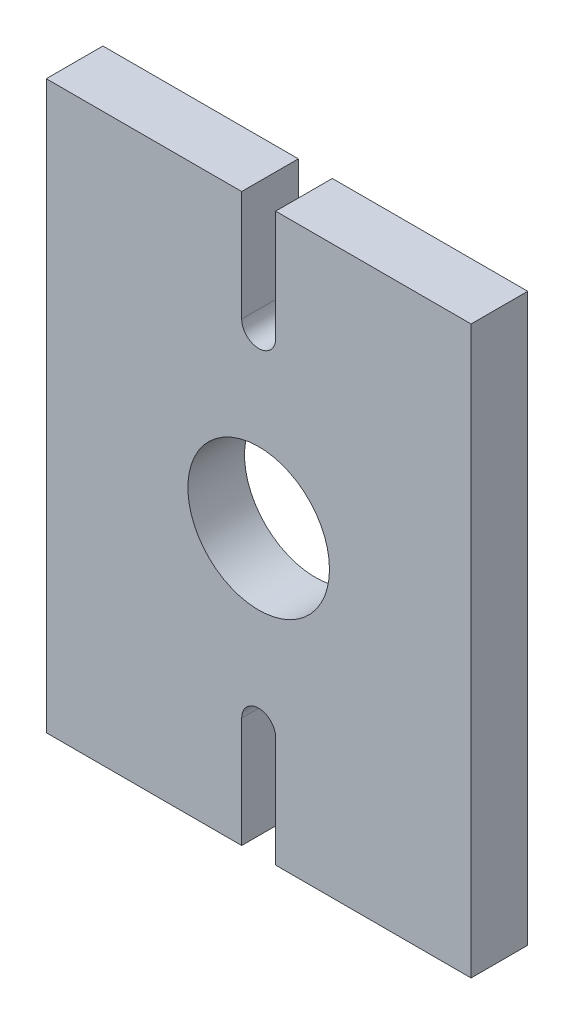
from build123d import *

# Parameters (mm, degrees)
SKETCH1_R           = 25
BOSS_EXTRUDE1_DEPTH = 20


with BuildPart() as part:
    # Sketch1 → Boss-Extrude1 (new body)
    with BuildSketch(Plane.XY):
        with BuildLine():
            Line((0, 0), (69, 0))
            Line((69, 0), (69, 39))
            ThreePointArc((69, 39), (75, 45), (81, 39))
            Line((81, 39), (81, 0))
            Line((81, 0), (150, 0))
            Line((150, 0), (150, 200))
            Line((150, 200), (81, 200))
            Line((81, 200), (81, 161))
            ThreePointArc((81, 161), (75, 155), (69, 161))
            Line((69, 161), (69, 200))
            Line((69, 200), (0, 200))
            Line((0, 200), (0, 0))
        make_face()
        with Locations((75, 100)):
            Circle(SKETCH1_R, mode=Mode.SUBTRACT)
    extrude(amount=BOSS_EXTRUDE1_DEPTH)


solid = part.part
